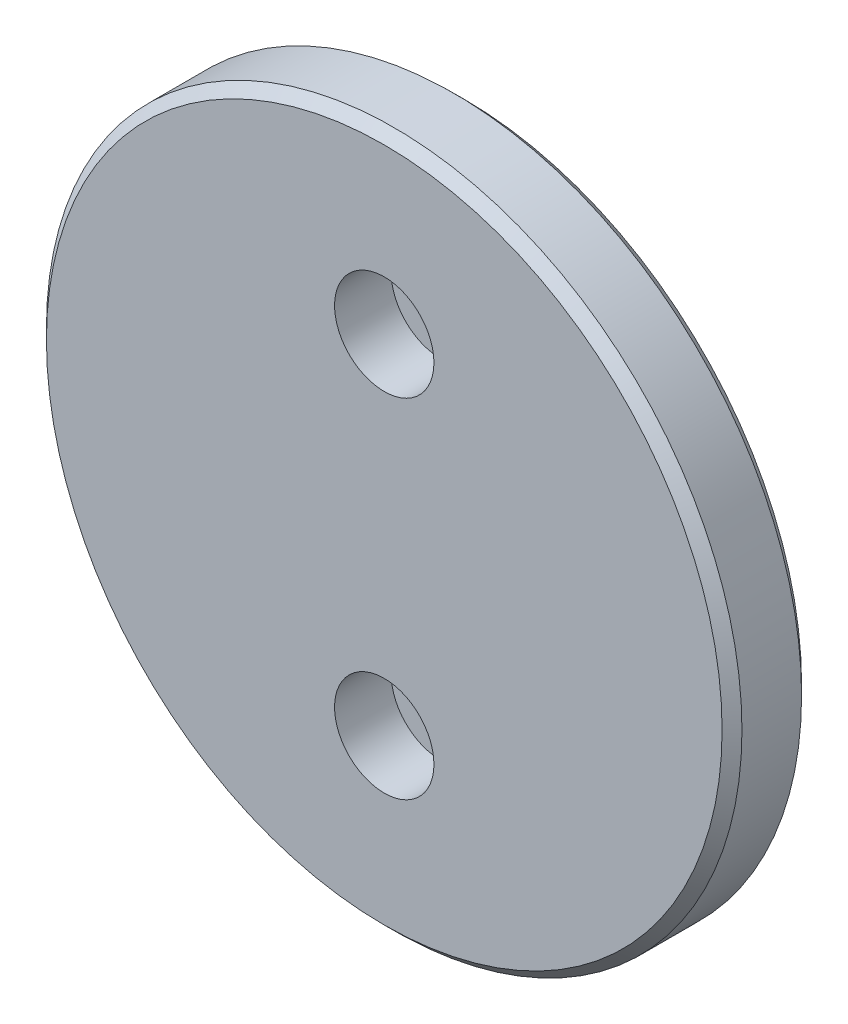
from build123d import *

# Parameters (mm, degrees)
SKETCH_1_R                = 35
EXTRUDE_1_DEPTH           = 8
HOLE_WIZARD_1_D           = 5.5
HOLE_WIZARD_1_CBORE_D     = 10
HOLE_WIZARD_1_CBORE_DEPTH = 5.7
CHAMFER_1_SIZE            = 1


with BuildPart() as part:
    # 草图1 → 凸台-拉伸1 (new body)
    with BuildSketch(Plane.XY):
        Circle(SKETCH_1_R)
    extrude(amount=EXTRUDE_1_DEPTH)

    # 打孔尺寸根据内六角圆柱头螺钉的类型1 (through all)
    with Locations(Plane.XY.offset(8)):
        with Locations((0, 17.5), (0, -17.5)):
            CounterBoreHole(HOLE_WIZARD_1_D / 2, HOLE_WIZARD_1_CBORE_D / 2, HOLE_WIZARD_1_CBORE_DEPTH)

    # 倒角1
    chamfer_1_edges = [part.edges().sort_by_distance(p)[0] for p in [
        (-35, 0, 0),
        (-35, 0, 8),
    ]]
    chamfer(chamfer_1_edges, length=CHAMFER_1_SIZE)


solid = part.part
